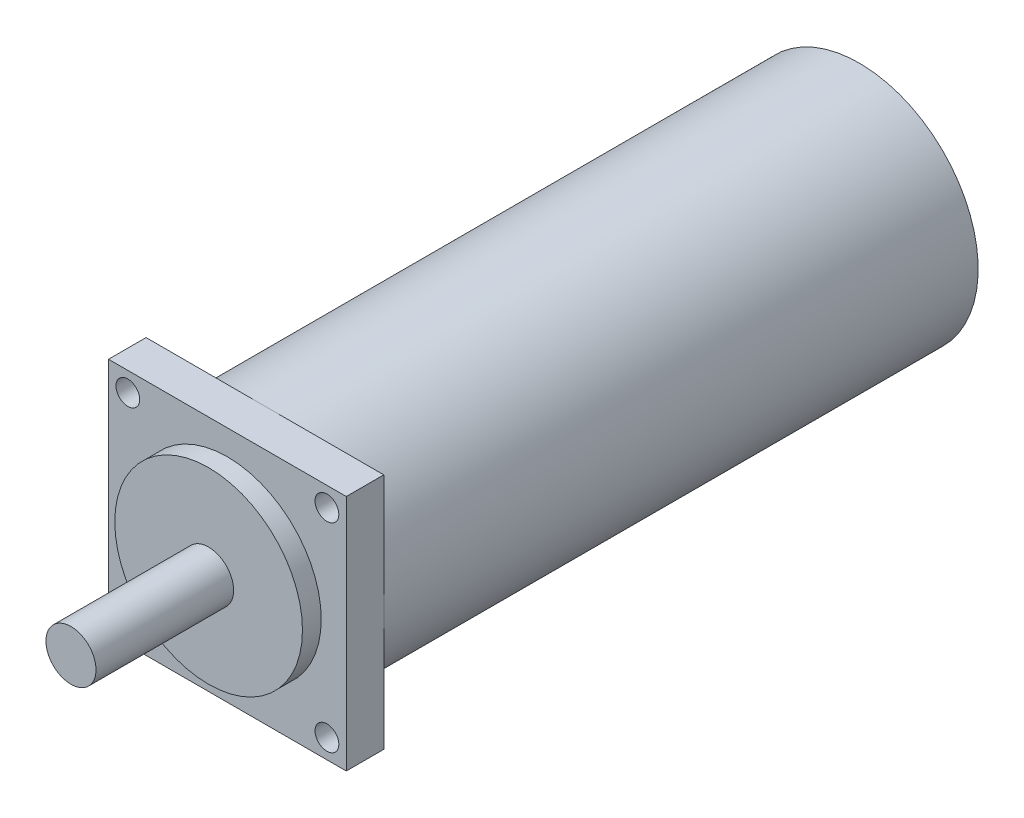
from build123d import *

# Parameters (mm, degrees)
SKETCH_1_W          = 38
SKETCH_1_H          = 38
EXTRUDE_1_DEPTH     = 6
SKETCH_2_R          = 15
EXTRUDE_2_DEPTH     = 3
SKETCH_3_R          = 4
EXTRUDE_3_DEPTH     = 22
SKETCH_4_R          = 19
EXTRUDE_4_DEPTH     = 97
CUT_EXTRUDE_1_REACH = 118.177
SKETCH_5_R          = 1.898690993
CHAMFER_1_SIZE      = 2
CHAMFER_1_SIZE2     = 4


with BuildPart() as part:
    # 草图1 → 拉伸1 (new body)
    with BuildSketch(Plane.XY):
        with Locations((19, 19)):
            Rectangle(SKETCH_1_W, SKETCH_1_H)
    extrude(amount=EXTRUDE_1_DEPTH)

    # 草图2 → 拉伸2 (add)
    with BuildSketch(Plane.XY.offset(6)):
        with Locations(Location((19, 19, 0), (0, 0, 180))):
            Circle(SKETCH_2_R)
    extrude(amount=EXTRUDE_2_DEPTH)

    # 草图3 → 拉伸3 (add)
    with BuildSketch(Plane.XY.offset(9)):
        with Locations((19, 19)):
            Circle(SKETCH_3_R)
    extrude(amount=EXTRUDE_3_DEPTH)

    # 草图4 → 拉伸4 (add)
    with BuildSketch(Plane(origin=(0, 0, 0), x_dir=(-1, 0, 0), z_dir=(0, 0, -1))):
        with Locations((-19, 19)):
            Circle(SKETCH_4_R)
    extrude(amount=EXTRUDE_4_DEPTH)

    # 草图5 → 切除-拉伸1 (cut, up to next)
    with BuildSketch(Plane.XY.offset(6), mode=Mode.PRIVATE) as cut_extrude_1_sk1:
        with Locations((3.090097423, 34.909902577)):
            Circle(SKETCH_5_R)
    cut_extrude_1_tool1 = extrude(cut_extrude_1_sk1.sketch, amount=-CUT_EXTRUDE_1_REACH, mode=Mode.PRIVATE) & part.part
    # 草图5 → 切除-拉伸1 (cut, up to next)
    with BuildSketch(Plane.XY.offset(6), mode=Mode.PRIVATE) as cut_extrude_1_sk2:
        with Locations((34.909902577, 34.909902577)):
            Circle(SKETCH_5_R)
    cut_extrude_1_tool2 = extrude(cut_extrude_1_sk2.sketch, amount=-CUT_EXTRUDE_1_REACH, mode=Mode.PRIVATE) & part.part
    # 草图5 → 切除-拉伸1 (cut, up to next)
    with BuildSketch(Plane.XY.offset(6), mode=Mode.PRIVATE) as cut_extrude_1_sk3:
        with Locations((34.909902577, 3.090097423)):
            Circle(SKETCH_5_R)
    cut_extrude_1_tool3 = extrude(cut_extrude_1_sk3.sketch, amount=-CUT_EXTRUDE_1_REACH, mode=Mode.PRIVATE) & part.part
    # 草图5 → 切除-拉伸1 (cut, up to next)
    with BuildSketch(Plane.XY.offset(6), mode=Mode.PRIVATE) as cut_extrude_1_sk4:
        with Locations((3.090097423, 3.090097423)):
            Circle(SKETCH_5_R)
    cut_extrude_1_tool4 = extrude(cut_extrude_1_sk4.sketch, amount=-CUT_EXTRUDE_1_REACH, mode=Mode.PRIVATE) & part.part
    add(cut_extrude_1_tool1.solids().sort_by_distance((3.090097, 34.909903, 6))[0], mode=Mode.SUBTRACT)
    add(cut_extrude_1_tool2.solids().sort_by_distance((34.909903, 34.909903, 6))[0], mode=Mode.SUBTRACT)
    add(cut_extrude_1_tool3.solids().sort_by_distance((34.909903, 3.090097, 6))[0], mode=Mode.SUBTRACT)
    add(cut_extrude_1_tool4.solids().sort_by_distance((3.090097, 3.090097, 6))[0], mode=Mode.SUBTRACT)

    # 倒角1
    chamfer_1_edges = [part.edges().sort_by_distance(p)[0] for p in [
        (38, 19, -97),
    ]]
    chamfer_1_side = [part.faces().sort_by_distance(p)[0] for p in [
        (38, 19, -48.5),
    ]]
    chamfer(chamfer_1_edges, length=CHAMFER_1_SIZE, length2=CHAMFER_1_SIZE2, reference=chamfer_1_side[0])


solid = part.part
